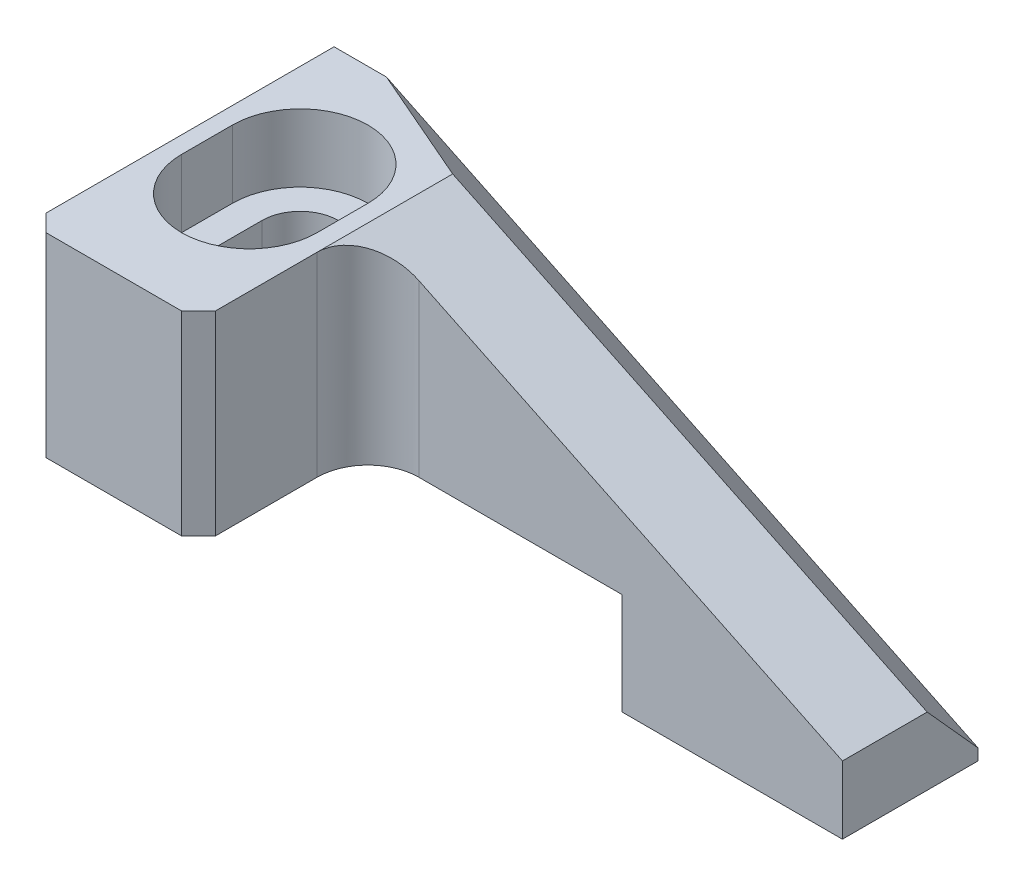
from build123d import *

# Parameters (mm, degrees)
BOSS_EXTRUDE1_DEPTH = 18
CHAMFER1_SIZE       = 3
CUT_EXTRUDE1_DEPTH  = 20
CUT_EXTRUDE3_DEPTH  = 4
SKETCH3_W           = 25
SKETCH3_H           = 6
CUT_EXTRUDE2_DEPTH  = 46.543934832
SKETCH5_W           = 28
SKETCH5_H           = 10
CUT_EXTRUDE4_DEPTH  = 46.543934832
FILLET1_R           = 3
CHAMFER2_SIZE       = 1


with BuildPart() as part:
    # Sketch1 → Boss-Extrude1 (new body)
    with BuildSketch(Plane.XY):
        Polygon((0, 17.5), (0, 0), (38, 0), (38, 4), (10, 17.5), align=None)
    extrude(amount=BOSS_EXTRUDE1_DEPTH)

    # Chamfer1
    chamfer1_edges = [part.edges().sort_by_distance(p)[0] for p in [
        (24, 10.75, 0),
    ]]
    chamfer(chamfer1_edges, length=CHAMFER1_SIZE)

    # Sketch2 → Cut-Extrude1 (cut)
    with BuildSketch(Plane(origin=(0, 17.5, 0), x_dir=(1, 0, 0), z_dir=(0, 1, 0))):
        with BuildLine():
            Line((2.75, -10), (2.75, -7))
            ThreePointArc((2.75, -7), (5, -4.75), (7.25, -7))
            Line((7.25, -7), (7.25, -10))
            ThreePointArc((7.25, -10), (5, -12.25), (2.75, -10))
        make_face()
    extrude(amount=-CUT_EXTRUDE1_DEPTH, mode=Mode.SUBTRACT)

    # Sketch4 → Cut-Extrude3 (cut)
    with BuildSketch(Plane(origin=(0, 17.5, 0), x_dir=(1, 0, 0), z_dir=(0, 1, 0))):
        with BuildLine():
            Line((9, -7), (9, -10))
            ThreePointArc((9, -10), (5, -14), (1, -10))
            Line((1, -10), (1, -7))
            ThreePointArc((1, -7), (5, -3), (9, -7))
        make_face()
    extrude(amount=-CUT_EXTRUDE3_DEPTH, mode=Mode.SUBTRACT)

    # Sketch3 → Cut-Extrude2 (cut, through all)
    with BuildSketch(Plane.XY.offset(18)):
        with Locations((12.5, 3)):
            Rectangle(SKETCH3_W, SKETCH3_H)
    extrude(amount=-CUT_EXTRUDE2_DEPTH, mode=Mode.SUBTRACT)

    # Sketch5 → Cut-Extrude4 (cut, through all)
    with BuildSketch(Plane(origin=(0, 17.5, 0), x_dir=(1, 0, 0), z_dir=(0, 1, 0))):
        with Locations((24, -13)):
            Rectangle(SKETCH5_W, SKETCH5_H)
    extrude(amount=-CUT_EXTRUDE4_DEPTH, mode=Mode.SUBTRACT)

    # Fillet1
    fillet1_edges = [part.edges().sort_by_distance(p)[0] for p in [
        (10, 11.75, 8),
    ]]
    fillet(fillet1_edges, radius=FILLET1_R)

    # Chamfer2
    chamfer2_edges = [part.edges().sort_by_distance(p)[0] for p in [
        (10, 11.75, 18),
        (0, 11.75, 18),
    ]]
    chamfer(chamfer2_edges, length=CHAMFER2_SIZE)


solid = part.part
